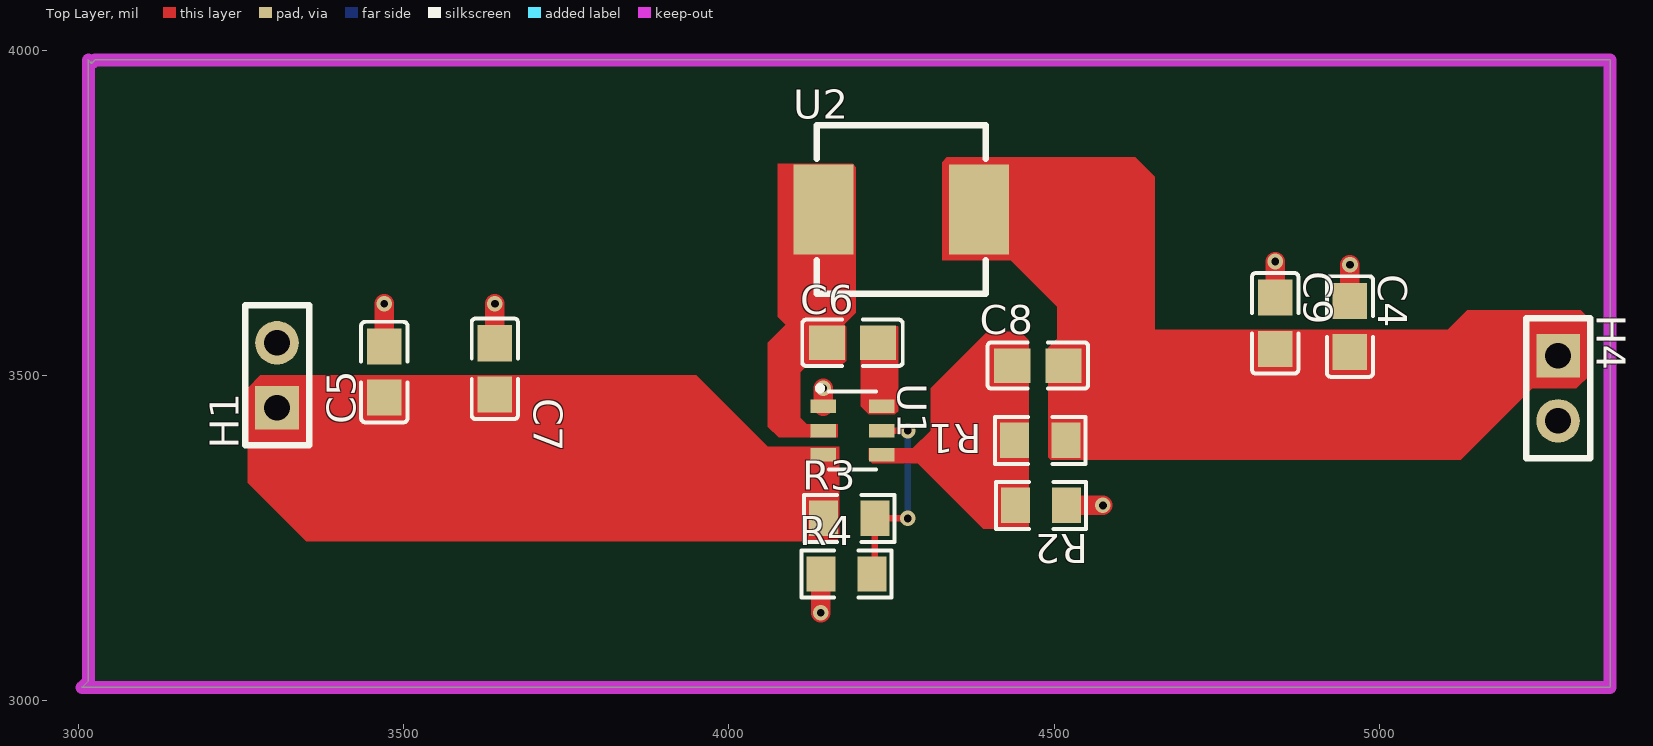
[diagram p0: Top Layer view]
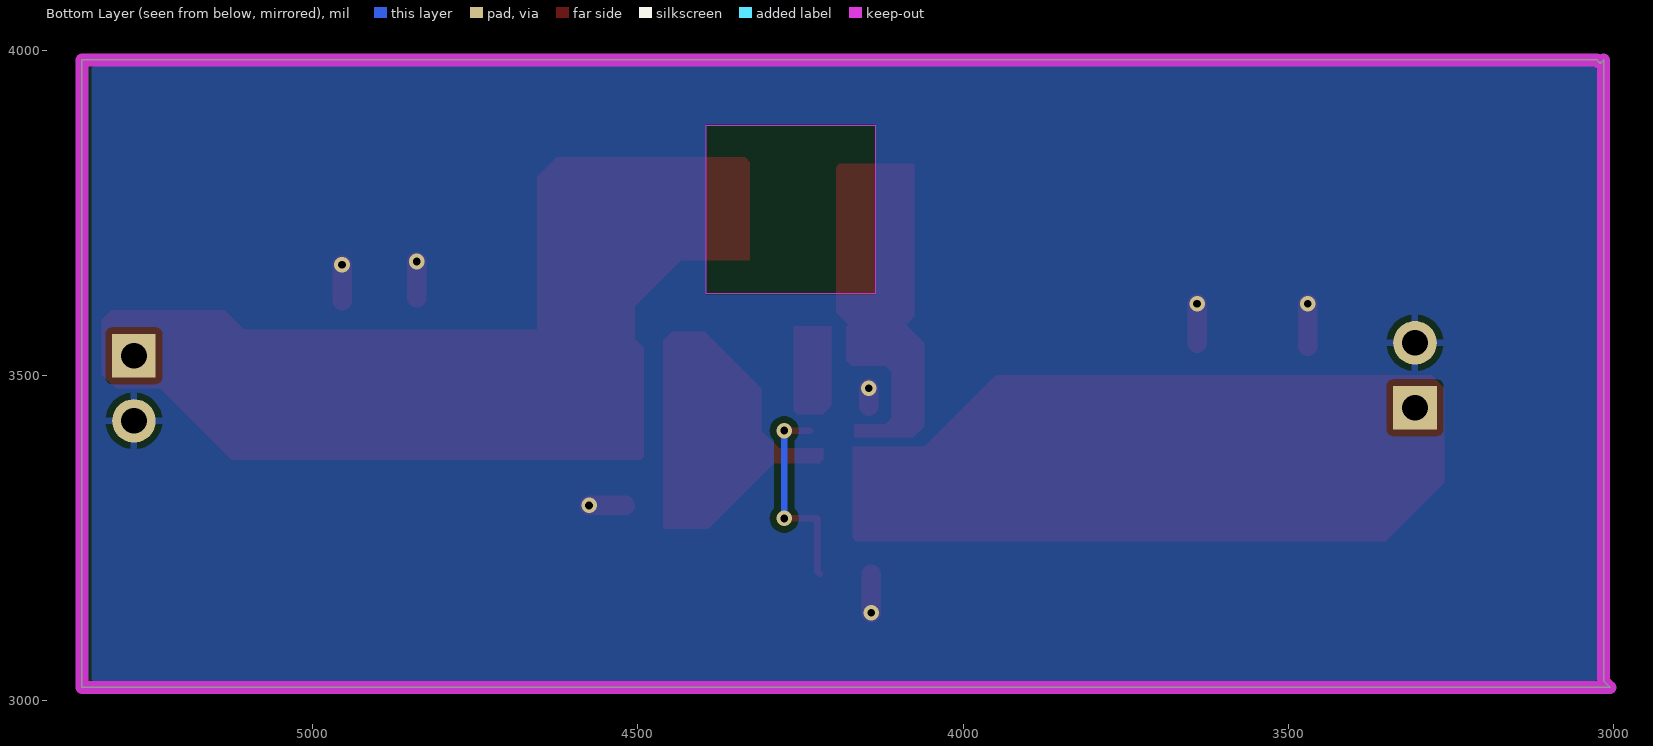
[diagram p1: Bottom Layer view, seen from below]
# Altium PCB MISC52146.pcbdoc
Units mil, origin at the board's own origin, x right, y up, seen from the top; angles counter-clockwise.
Board outline 2350 x 965 mil, 2 copper layers (Top Layer, Bottom Layer), stack 62.206 mil thick; 14 components, 7 nets, 32 pads, 9 vias.

## Layer stack, top to bottom
Top Solder Mask Layer: solder mask 0.394, Dk 3.3
Top Layer: signal copper 1.379
Dielectric1: surface 59.449, FR4, Dk 4.5
Bottom Layer: signal copper 1.378
Bottom Solder Mask Layer: solder mask 0.394, Dk 3.3

## Board outline
3015,3985 3015,3030 3005,3020 5355,3020 5355,3985 3025,3985 3020,3980

## Design rules (kind name [scope] priority, off if disabled: settings)
BoardOutlineClearance copperThickness2oz_1 [All] p2 off: genericclearance=7.99 ignorepadtopadclearanceinfootprint=FALSE except(0: Arc-SplitContinuation Track-SplitContinuation SMDPad-SplitContinuation THPad-SplitContinuation Via-SplitContinuation Fill-SplitContinuation Region-SplitContinuation Poly-SplitContinuation Text-SplitContinuation Hole-SplitContinuation; 5.98: Arc-CutoutEdge Track-CutoutEdge SMDPad-CutoutEdge THPad-CutoutEdge Via-CutoutEdge Text-CutoutEdge; 6.9: Hole-OutlineEdge Hole-CutoutEdge; 10: Poly-OutlineEdge Poly-CutoutEdge; 11.81: Arc-OutlineEdge Track-OutlineEdge SMDPad-OutlineEdge THPad-OutlineEdge Via-OutlineEdge Fill-OutlineEdge Region-OutlineEdge Text-OutlineEdge Fill-CutoutEdge Region-CutoutEdge)
BoardOutlineClearance Plane_innerPlane_1 [All] p4 off: genericclearance=4.02 ignorepadtopadclearanceinfootprint=FALSE except(0: Arc-SplitContinuation Track-SplitContinuation SMDPad-SplitContinuation THPad-SplitContinuation Via-SplitContinuation Fill-SplitContinuation Region-SplitContinuation Poly-SplitContinuation Text-SplitContinuation Hole-SplitContinuation; 5.98: Arc-CutoutEdge Track-CutoutEdge SMDPad-CutoutEdge THPad-CutoutEdge Via-CutoutEdge Text-CutoutEdge; 6.9: Hole-OutlineEdge Hole-CutoutEdge; 10: Poly-OutlineEdge Poly-CutoutEdge; 11.81: Arc-OutlineEdge Track-OutlineEdge SMDPad-OutlineEdge THPad-OutlineEdge Via-OutlineEdge Fill-OutlineEdge Region-OutlineEdge Text-OutlineEdge Fill-CutoutEdge Region-CutoutEdge)
BoardOutlineClearance Copper_copperRegion_1 [All] p6 off: genericclearance=4.02 ignorepadtopadclearanceinfootprint=FALSE except(0: Arc-SplitContinuation Track-SplitContinuation SMDPad-SplitContinuation THPad-SplitContinuation Via-SplitContinuation Fill-SplitContinuation Region-SplitContinuation Poly-SplitContinuation Text-SplitContinuation Hole-SplitContinuation; 5.98: Arc-CutoutEdge Track-CutoutEdge SMDPad-CutoutEdge THPad-CutoutEdge Via-CutoutEdge Text-CutoutEdge; 6.9: Hole-OutlineEdge Hole-CutoutEdge; 10: Poly-OutlineEdge Poly-CutoutEdge; 11.81: Arc-OutlineEdge Track-OutlineEdge SMDPad-OutlineEdge THPad-OutlineEdge Via-OutlineEdge Fill-OutlineEdge Region-OutlineEdge Text-OutlineEdge Fill-CutoutEdge Region-CutoutEdge)
BoardOutlineClearance copperThickness1oz_1 [All] p8: genericclearance=4.02 ignorepadtopadclearanceinfootprint=FALSE except(0: Arc-SplitContinuation Track-SplitContinuation SMDPad-SplitContinuation THPad-SplitContinuation Via-SplitContinuation Fill-SplitContinuation Region-SplitContinuation Poly-SplitContinuation Text-SplitContinuation Hole-SplitContinuation; 5.98: Arc-CutoutEdge Track-CutoutEdge SMDPad-CutoutEdge THPad-CutoutEdge Via-CutoutEdge Text-CutoutEdge; 6.9: Hole-OutlineEdge Hole-CutoutEdge; 10: Poly-OutlineEdge Poly-CutoutEdge; 11.81: Arc-OutlineEdge Track-OutlineEdge SMDPad-OutlineEdge THPad-OutlineEdge Via-OutlineEdge Fill-OutlineEdge Region-OutlineEdge Text-OutlineEdge Fill-CutoutEdge Region-CutoutEdge)
Clearance copperThickness2oz [All] p1 off: gap=7.99 ignorepadtopadclearanceinfootprint=FALSE except(5.98: SMDPad-Track SMDPad-SMDPad THPad-Track SMDPad-THPad THPad-THPad Track-Via SMDPad-Via THPad-Via Via-Via Fill-SMDPad Region-SMDPad Fill-THPad Region-THPad Fill-Via Region-Via Fill-Fill Fill-Region Region-Region Arc-Track Arc-SMDPad Arc-THPad Arc-Via Fill-Arc Region-Arc Arc-Arc Text-Track SMDPad-Text Text-THPad Text-Via Fill-Text Region-Text Arc-Text Text-Text; 6.9: Hole-Track Hole-SMDPad Hole-THPad Hole-Via Fill-Hole Region-Hole Hole-Arc Hole-Text; 10: Poly-Track Poly-SMDPad Poly-THPad Poly-Via Poly-Fill Poly-Region Poly-Poly Poly-Arc Poly-Text Poly-Hole; 11.81: Fill-Track Region-Track)
Clearance Plane_innerPlane [All] p3 off: gap=4.02 ignorepadtopadclearanceinfootprint=FALSE except(5.98: SMDPad-Track SMDPad-SMDPad THPad-Track SMDPad-THPad THPad-THPad Track-Via SMDPad-Via THPad-Via Via-Via Fill-SMDPad Region-SMDPad Fill-THPad Region-THPad Fill-Via Region-Via Fill-Fill Fill-Region Region-Region Arc-Track Arc-SMDPad Arc-THPad Arc-Via Fill-Arc Region-Arc Arc-Arc Text-Track SMDPad-Text Text-THPad Text-Via Fill-Text Region-Text Arc-Text Text-Text; 6.9: Hole-Track Hole-SMDPad Hole-THPad Hole-Via Fill-Hole Region-Hole Hole-Arc Hole-Text; 10: Poly-Track Poly-SMDPad Poly-THPad Poly-Via Poly-Fill Poly-Region Poly-Poly Poly-Arc Poly-Text Poly-Hole; 11.81: Fill-Track Region-Track)
Clearance Copper_copperRegion [All] p5 off: gap=4.02 ignorepadtopadclearanceinfootprint=FALSE except(5.98: SMDPad-Track SMDPad-SMDPad THPad-Track SMDPad-THPad THPad-THPad Track-Via SMDPad-Via THPad-Via Via-Via Fill-SMDPad Region-SMDPad Fill-THPad Region-THPad Fill-Via Region-Via Fill-Fill Fill-Region Region-Region Arc-Track Arc-SMDPad Arc-THPad Arc-Via Fill-Arc Region-Arc Arc-Arc Text-Track SMDPad-Text Text-THPad Text-Via Fill-Text Region-Text Arc-Text Text-Text; 6.9: Hole-Track Hole-SMDPad Hole-THPad Hole-Via Fill-Hole Region-Hole Hole-Arc Hole-Text; 10: Poly-Track Poly-SMDPad Poly-THPad Poly-Via Poly-Fill Poly-Region Poly-Poly Poly-Arc Poly-Text Poly-Hole; 11.81: Fill-Track Region-Track)
Clearance copperThickness1oz [All] p7: gap=4.02 ignorepadtopadclearanceinfootprint=FALSE except(5.98: SMDPad-Track SMDPad-SMDPad THPad-Track SMDPad-THPad THPad-THPad Track-Via SMDPad-Via THPad-Via Via-Via Fill-SMDPad Region-SMDPad Fill-THPad Region-THPad Fill-Via Region-Via Fill-Fill Fill-Region Region-Region Arc-Track Arc-SMDPad Arc-THPad Arc-Via Fill-Arc Region-Arc Arc-Arc Text-Track SMDPad-Text Text-THPad Text-Via Fill-Text Region-Text Arc-Text Text-Text; 6.9: Hole-Track Hole-SMDPad Hole-THPad Hole-Via Fill-Hole Region-Hole Hole-Arc Hole-Text; 10: Poly-Track Poly-SMDPad Poly-THPad Poly-Via Poly-Fill Poly-Region Poly-Poly Poly-Arc Poly-Text Poly-Hole; 11.81: Fill-Track Region-Track)
DiffPairsRouting differentialPair [All] p1: maxlimit=6 minlimit=6 mostfreqgap=6 toplayer_minwidth=5 toplayer_prefwidth=10 toplayer_maxwidth=100 toplayer_mingap=6 toplayer_prefgap=6 toplayer_maxgap=6 bottomlayer_minwidth=5 bottomlayer_prefwidth=10 bottomlayer_maxwidth=100 bottomlayer_mingap=6 bottomlayer_prefgap=6 bottomlayer_maxgap=6 maxuncoupledlength=10
HoleToHoleClearance otherClearance [All] p1: gap=11.81 allowstackedmicrovias=TRUE
Length netLength [All] p1: minlimit=0 maxlimit=0
PasteMaskExpansion pasteMaskExpansion [All] p1: expansion=0
PlaneConnect innerPlane [All] p1: planeconnectstyle=Relief reliefexpansion=20 reliefentries=4 reliefconductorwidth=10 reliefairgap=10
PolygonConnect copperRegion [All] p1: connectstyle=Relief reliefconductorwidth=10 reliefentries=4 polygonreliefangle="90 Angle" airgapwidth=10 via.connectstyle=Relief via.reliefconductorwidth=10 via.reliefentries=4 via.polygonreliefangle="90 Angle" via.airgapwidth=10
RoutingVias viaSize [All] p1: holewidth=12.01 width=24.02 viastyle="Through Hole" minholewidth=11.81 minwidth=19.68 maxholewidth=248.03 maxwidth=393.7
SolderMaskExpansion solderMaskExpansion [IsVia] p1: expansion=-1000 istentingtop=TRUE
SolderMaskExpansion solderMaskExpansion [All] p2: expansion=2 istentingtop=FALSE
Width copperThickness2oz_2 [All] p1 off: maxlimit=100 minlimit=8 preferedwidth=10
Width copperThickness1oz_2 [All] p2: maxlimit=100 minlimit=5 preferedwidth=10

## Components (designator, comment, footprint, x,y, rotation, side; value= is the part's Value field where it differs from the comment)
C4 "22uF" C0805 4955,3575 r270 top
C5 "10uF" C0805 3470,3505 r90 top
C6 "100nF" C0805 4190,3550 r0 top
C7 "0.1uF" C0805 3640,3510 r270 top
C8 "75pF" C0805 4475,3515 r0 top
C9 "22uF" C0805 4840,3580 r270 top
H1 "电源输入" HDR-TH_2P-P2.54-V-F 3305,3500 r90 top
H4 "电源输出" HDR-TH_2P-P2.54-V-F 5275,3480 r270 top
R1 "100k" R0805 4478.74,3400 r0 top
R2 "13300" R0805 4480,3300 r180 top
R3 "511k" R0805 4185,3280 r0 top
R4 "105K" R0805 4180.63,3194.37 r0 top
U1 "GD30DC1354" SOT-23-6_L2.9-W1.7-P0.95-LS2.8-BL 4190,3415 r270 top
U2 "15uH" IND-SMD_L6.6-W6.6 4265,3755 r0 top

## Footprints (in the part's own frame and the unit in brackets; to place one, negate y for a bottom-side part, rotate by r counter-clockwise, add the part's x,y. Pads: shape width x height; smd on the part's side, far side on the other; paste and mask are expansions set on the pad)
C0805 [mm]
  rect 1.41x1.35 smd paste-100 mask+0.051: 1(-1,0) 2(1,0)
  silkscreen extent -1.96,-0.9 1.96,0.9
HDR-TH_2P-P2.54-V-F [mm]
  rect 1.7x1.7 hole 1: 1(-1.27,0)
  round 1.7 hole 1: 2(1.27,0)
  silkscreen extent -2.74,-1.25 2.74,1.25
IND-SMD_L6.6-W6.6 [mm]
  rect 2.35x3.5 smd: 1(-3.035,0) 2(3.035,0)
  silkscreen extent -3.3,-3.3 3.3,3.3
R0805 [mm]
  rect 1.133x1.377 smd paste-100 mask+0.051: 1(-1,0) 2(1,0)
  silkscreen extent -1.76,-0.92 1.76,0.92
SOT-23-6_L2.9-W1.7-P0.95-LS2.8-BL [mm]
  rect 0.532x0.99 smd: 1(-0.95,-1.145) 2(0,-1.145) 3(0.95,-1.145) 4(0.95,1.145) 5(0,1.145) 6(-0.95,1.145)
  silkscreen extent -1.75,-1.37 1.53,0.93

## Via types
v1: diameter 24.02, hole 12, Top Layer to Bottom Layer, 9 vias

## Nets (pads, with @x,y where several pads share a name; then routed paths per layer and width w, separated by ;. In a path a pad name is that pad's centre, name@x,y a point inside that pad or via, vN(x,y) a via of type N, cw(c..) or ccw(c..) an arc to the next point about the centre after c; other vN are vias at no path point)
$1N502: C4.2 C8.2 C9.2 H4.1 R1.2 U2.2
$1N1606: R3.2 R4.2 U1.5 | length 313
  Top Layer w10: R4.2 4224.37,3198.74 R3.2 v1(4275,3280) ; U1.5 v1(4275,3415)
  Bottom Layer w10: v1(4275,3280) v1(4275,3415)
$1N1610: C8.1 R1.1 R2.2 U1.4
$1N1625: C6.2 U1.6
$1N1648: C6.1 U1.2 U2.1
$1N1666: C5.1 C7.2 H1.1 R3.1 U1.3
GND: C4.1 C5.2 C7.1 C9.1 H1.2 H4.2 R2.1 R4.1 U1.1 | length 380.2
  Top Layer w30: C5.2 v1(3470,3610) ; C7.1 v1(3640,3610) ; v1(4141.26,3135) R4.1 ; U1.1 4145,3452.48 v1(4145,3480) ; R2.1 v1(4575,3300) ; C9.1 v1(4840,3675) ; C4.1 v1(4955,3670)

## Polygon pours and split planes (outlines as drawn)
GND on Bottom Layer (solid, remove dead copper, pour order 0): 3000,4033.74 3000,3000 5340,3000 5340,4033.74

## Keep-outs
Bottom Layer:
  region: 4135.08,3884.92 4135.08,3625.08 4394.92,3625.08 4394.92,3884.92
Board Outline Layer:
  the board outline again, w20

## Other copper
Top Layer:
  region net $1N1610: 4459.22,3554.22 4460,3555 4460.78,3554.22
  region net $1N1610: 4397.27,3567.27 4447.73,3567.27 4461.25,3553.75 4461.25,3263.89 4391.11,3263.89 4290,3365 4220,3365 4215,3370 4215,3387.52 4282.52,3387.52 4310,3415 4310,3480
  region net $1N1610: 4455.57,3550.57 4403.69,3550.57 4407.34,3554.22 4459.22,3554.22
  region net $1N1666: 4170,3390 4170,3250 4165,3245 3350,3245 3260,3335 3260,3480.48 3279.52,3500 3950,3500 4060,3390
  region net $1N502: 4490.94,3542.17 4518.78,3570 5105,3570 5135,3600 5310,3600 5324.21,3585.79 5324.21,3501.22 5302.99,3480 5235,3480 5125,3370 4495,3370 4490.94,3374.06
  region net $1N502: 4335,3835 4625,3835 4655,3805 4655,3550 4640,3535 4525.94,3535 4504.86,3556.08 4504.86,3605.14 4433,3677 4327.98,3677 4327.98,3827.98
  region net $1N1648: 4173.58,3581.42 4180,3575 4180,3522.53 4171.89,3514.43 4119.43,3514.43 4110,3505 4110,3435 4120,3425 4167.41,3425 4167.41,3404.44 4076.55,3404.44 4060,3420.98 4060,3550 4091.42,3581.42
  region net $1N1625: 4202.91,3575.2 4259.8,3575.2 4260,3575 4260,3445 4255,3440 4215,3440 4202.91,3452.09
  region net $1N1648: 4190,3825 4195,3820 4195,3596.42 4175,3576.42 4088.91,3576.42 4075,3590.32 4075,3825